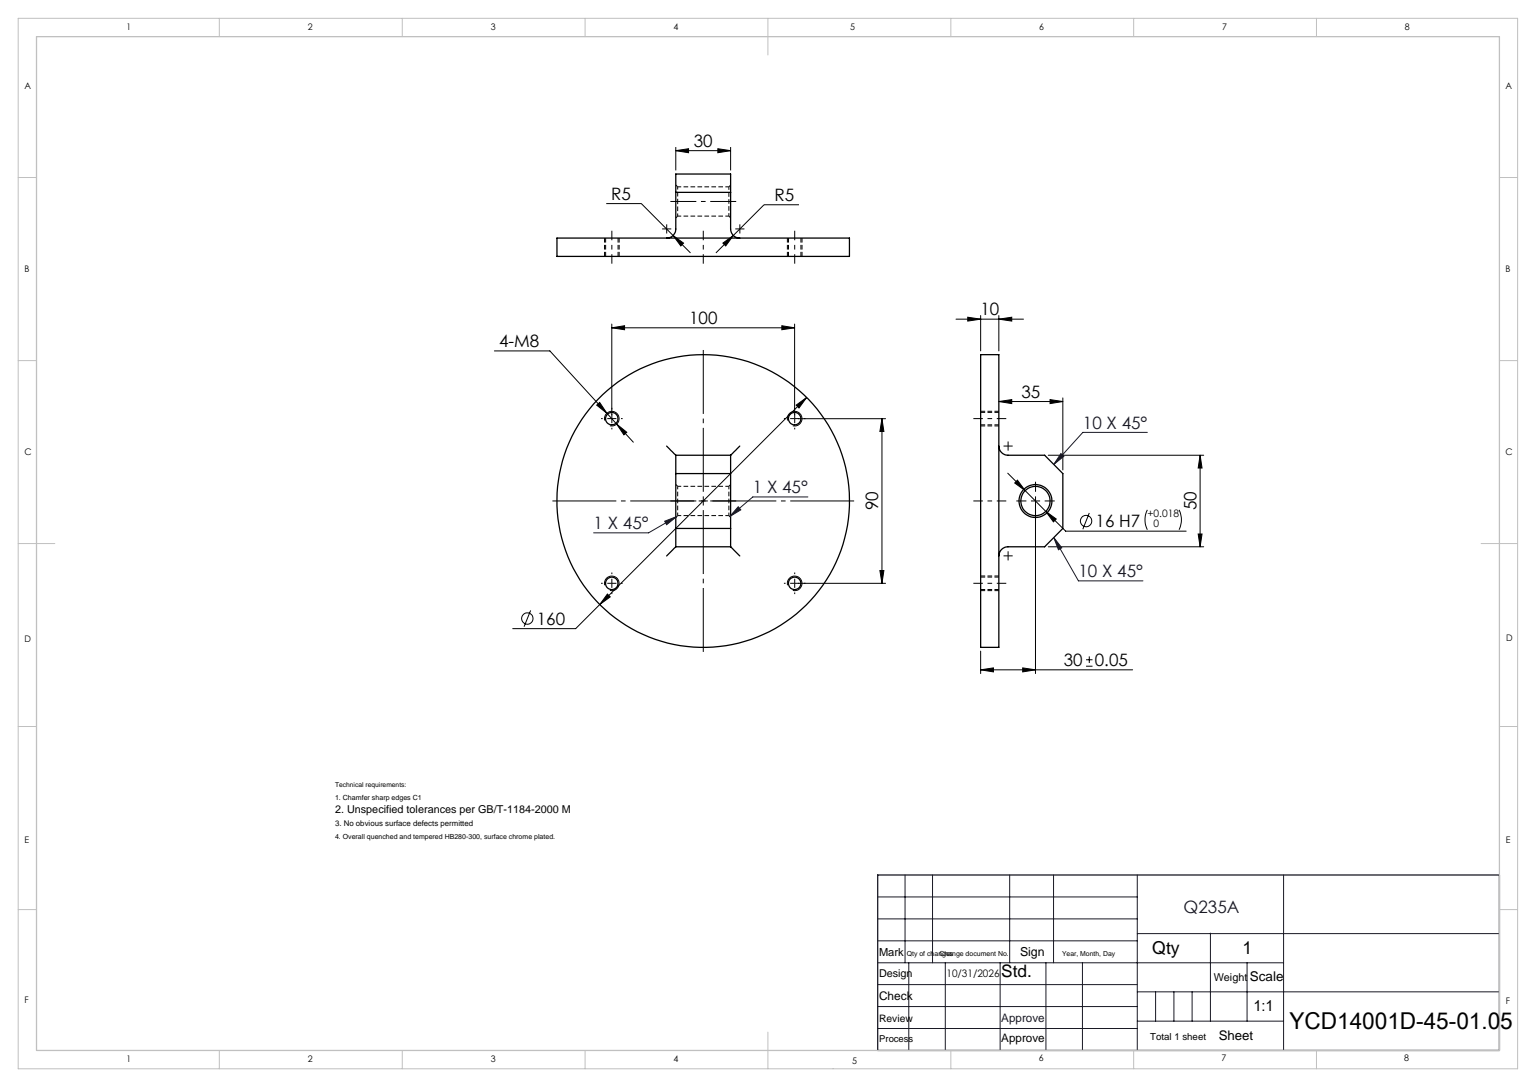
from build123d import *

# Parameters (mm, degrees)
SKETCH1_R           = 80
BOSS_EXTRUDE1_DEPTH = 5
M8_TAPPED_HOLE1_D   = 6.8
SKETCH7_W           = 30
SKETCH7_H           = 50
BOSS_EXTRUDE2_DEPTH = 35
SKETCH8_R           = 8
CUT_EXTRUDE4_DEPTH  = 131.479883507
CHAMFER1_SIZE       = 10
FILLET3_R           = 5
CHAMFER2_SIZE       = 1


with BuildPart() as part:
    # Sketch1 → Boss-Extrude1 (new, symmetric)
    with BuildSketch(Plane(origin=(0, 0, 0), x_dir=(1, 0, 0), z_dir=(0, 1, 0))):
        with Locations(Location((0, 0, 0), (0, 0, 270))):
            Circle(SKETCH1_R)
    extrude(amount=BOSS_EXTRUDE1_DEPTH, both=True)

    # M8 Tapped Hole1 (through all)
    with Locations(Plane(origin=(0, -5, 0), x_dir=(-1, 0, 0), z_dir=(0, -1, 0))):
        with Locations((50, -45), (50, 45), (-50, 45), (-50, -45)):
            Hole(M8_TAPPED_HOLE1_D / 2)

    # Sketch7 → Boss-Extrude2 (add)
    with BuildSketch(Plane.XZ.offset(5)):
        Rectangle(SKETCH7_W, SKETCH7_H)
    extrude(amount=BOSS_EXTRUDE2_DEPTH)

    # Sketch8 → Cut-Extrude4 (cut, through all)
    with BuildSketch(Plane(origin=(15, 0, 0), x_dir=(0, 0, -1), z_dir=(1, 0, 0))):
        with Locations((0, -25)):
            Circle(SKETCH8_R)
    extrude(amount=-CUT_EXTRUDE4_DEPTH, mode=Mode.SUBTRACT)

    # Chamfer1
    chamfer1_edges = [part.edges().sort_by_distance(p)[0] for p in [
        (0, -40, 25),
        (0, -40, -25),
    ]]
    chamfer(chamfer1_edges, length=CHAMFER1_SIZE)

    # Fillet3
    fillet3_edges = [part.edges().sort_by_distance(p)[0] for p in [
        (15, -5, 0),
        (0, -5, 25),
        (-15, -5, 0),
        (0, -5, -25),
    ]]
    fillet(fillet3_edges, radius=FILLET3_R)

    # Chamfer2
    chamfer2_edges = [part.edges().sort_by_distance(p)[0] for p in [
        (-15, -25, 8),
        (15, -25, 8),
    ]]
    chamfer(chamfer2_edges, length=CHAMFER2_SIZE)


solid = part.part
